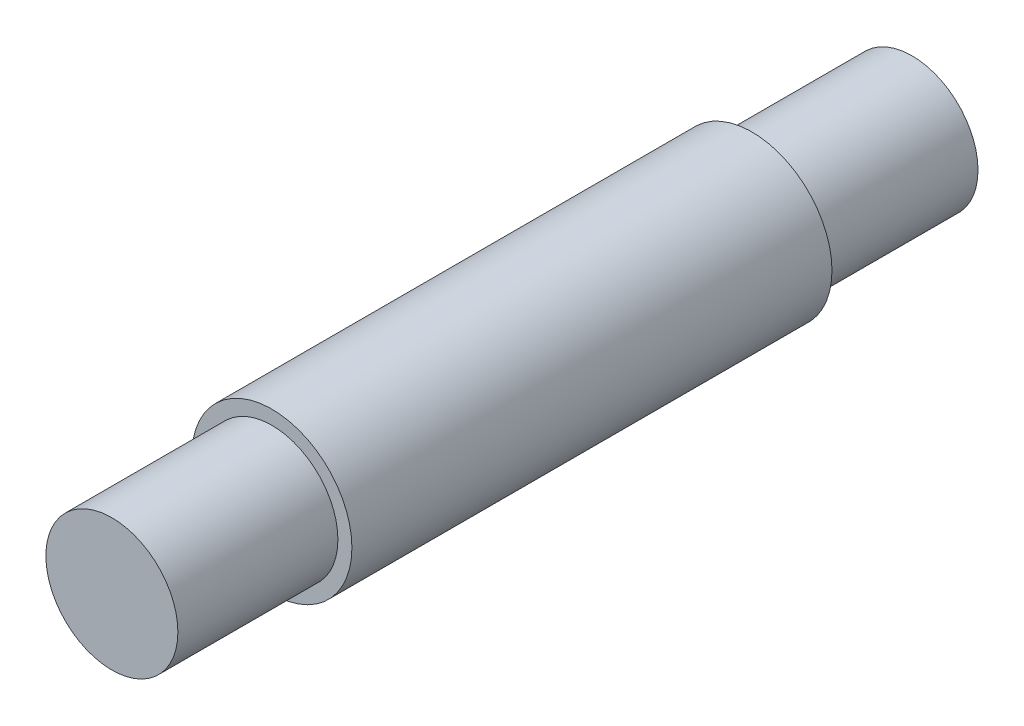
from build123d import *

# Parameters (mm, degrees)
SKETCH_1_R           = 20
BOSS_EXTRUDE_1_DEPTH = 60
SKETCH_2_R           = 16.5
BOSS_EXTRUDE_2_DEPTH = 40


with BuildPart() as part:
    # Sketch 1 → Boss-Extrude 1 (new, symmetric)
    with BuildSketch(Plane.XY):
        Circle(SKETCH_1_R)
    extrude(amount=BOSS_EXTRUDE_1_DEPTH, both=True)

    # Sketch 2 → Boss-Extrude 2 (add)
    with BuildSketch(Plane.XY.offset(60)):
        Circle(SKETCH_2_R)
    boss_extrude_2 = extrude(amount=BOSS_EXTRUDE_2_DEPTH)

    # Mirror 1: Boss-Extrude 2 across plane
    add(boss_extrude_2.mirror(Plane.XY))


solid = part.part
